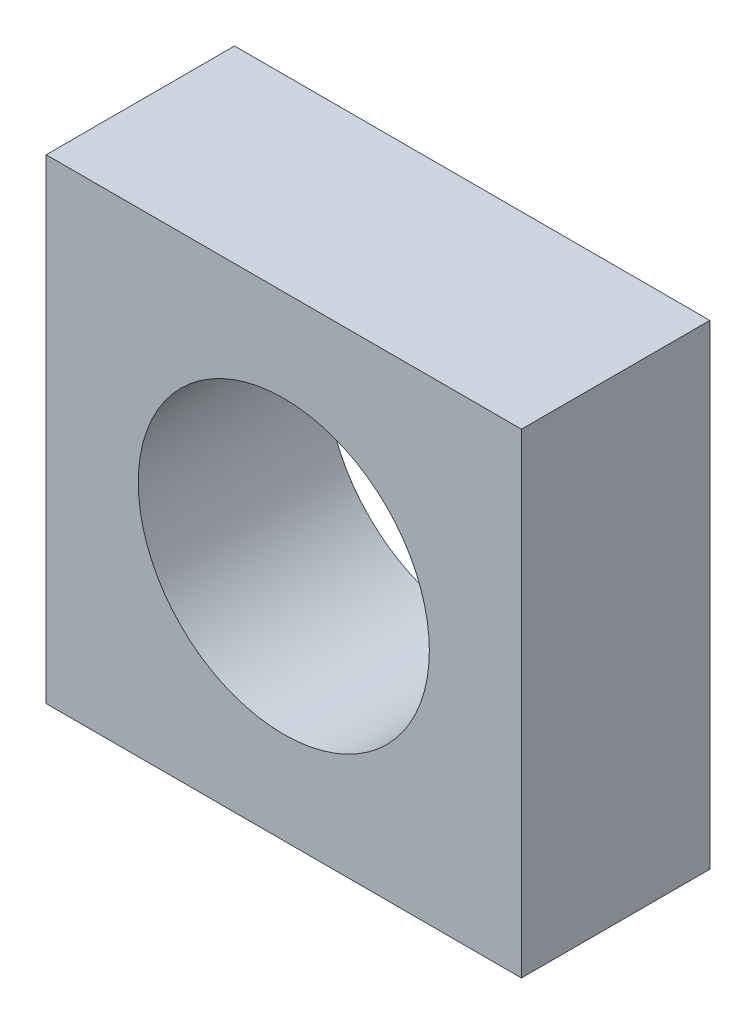
from build123d import *

# Parameters (mm, degrees)
SKETCH1_W           = 12
SKETCH1_H           = 12
SKETCH1_R           = 3.674588618
BOSS_EXTRUDE1_DEPTH = 4.755965796


with BuildPart() as part:
    # Sketch1 → Boss-Extrude1 (new body)
    with BuildSketch(Plane.XY):
        with Locations((19.551834603, 1.836555855)):
            Rectangle(SKETCH1_W, SKETCH1_H)
        with Locations((19.551834603, 1.836555855)):
            Circle(SKETCH1_R, mode=Mode.SUBTRACT)
    extrude(amount=BOSS_EXTRUDE1_DEPTH)


solid = part.part
